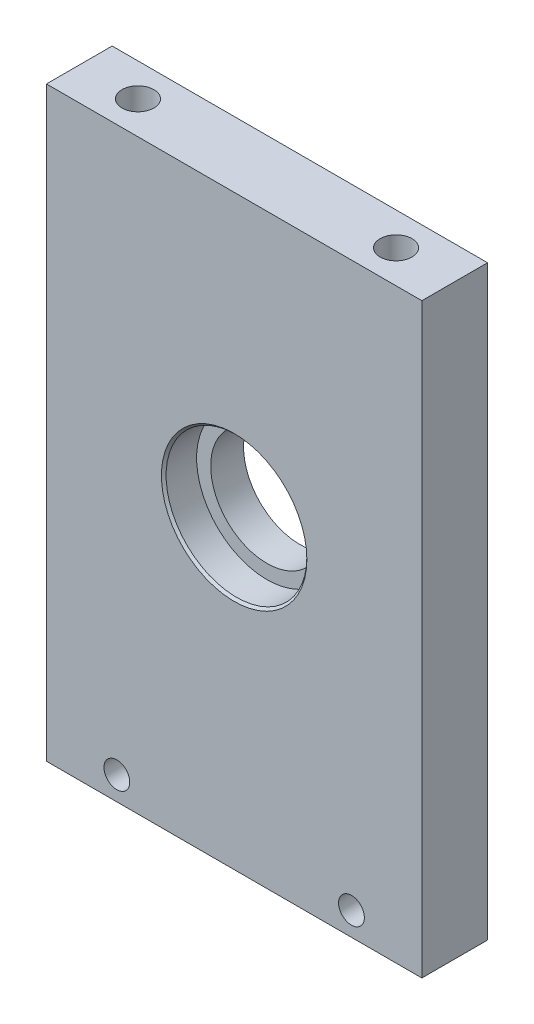
from build123d import *

# Parameters (mm, degrees)
SKETCH_1_W             = 80
SKETCH_1_H             = 125
EXTRUDE_1_DEPTH        = 14
SKETCH_2_R             = 15
CUT_EXTRUDE_1_DEPTH    = 7
SKETCH_3_R             = 12
CUT_EXTRUDE_2_DEPTH    = 149.573214275
CHAMFER_2_SIZE         = 0.5
HOLE_WIZARD_M8_1_D     = 6.8
HOLE_WIZARD_M8_1_DEPTH = 22.25
HOLE_WIZARD_M8_1_TIP   = 2.042926105
SKETCH_10_R            = 2.75
CUT_EXTRUDE_3_DEPTH    = 150.067098986


with BuildPart() as part:
    # 草图1 → 凸台-拉伸1 (new body)
    with BuildSketch(Plane.XY):
        with Locations((40, -62.5)):
            Rectangle(SKETCH_1_W, SKETCH_1_H)
    extrude(amount=EXTRUDE_1_DEPTH)

    # 草图2 → 切除-拉伸1 (cut)
    with BuildSketch(Plane.XY.offset(14)):
        with Locations((40, -60)):
            Circle(SKETCH_2_R)
    extrude(amount=-CUT_EXTRUDE_1_DEPTH, mode=Mode.SUBTRACT)

    # 草图3 → 切除-拉伸2 (cut, through all)
    with BuildSketch(Plane.XY.offset(7)):
        with Locations((40, -60)):
            Circle(SKETCH_3_R)
    extrude(amount=-CUT_EXTRUDE_2_DEPTH, mode=Mode.SUBTRACT)

    # 倒角2
    chamfer_2_edges = [part.edges().sort_by_distance(p)[0] for p in [
        (25, -60, 14),
    ]]
    chamfer(chamfer_2_edges, length=CHAMFER_2_SIZE)

    # M8 螺纹孔1
    with Locations(Plane(origin=(0, 0, 0), x_dir=(1, 0, 0), z_dir=(0, 1, 0))):
        with Locations((67.5, -7), (12.5, -7)):
            Hole(HOLE_WIZARD_M8_1_D / 2, depth=HOLE_WIZARD_M8_1_DEPTH)
            with Locations((0, 0, -(HOLE_WIZARD_M8_1_DEPTH + HOLE_WIZARD_M8_1_TIP / 2))):  # 118° drill point
                Cone(0, HOLE_WIZARD_M8_1_D / 2, HOLE_WIZARD_M8_1_TIP, mode=Mode.SUBTRACT)

    # 草图10 → 切除-拉伸3 (cut, through all)
    with BuildSketch(Plane(origin=(0, 0, 0), x_dir=(-1, 0, 0), z_dir=(0, 0, -1))):
        with Locations((-65, -120)):
            Circle(SKETCH_10_R)
        with Locations((-15, -120)):
            Circle(SKETCH_10_R)
    extrude(amount=-CUT_EXTRUDE_3_DEPTH, mode=Mode.SUBTRACT)


solid = part.part
